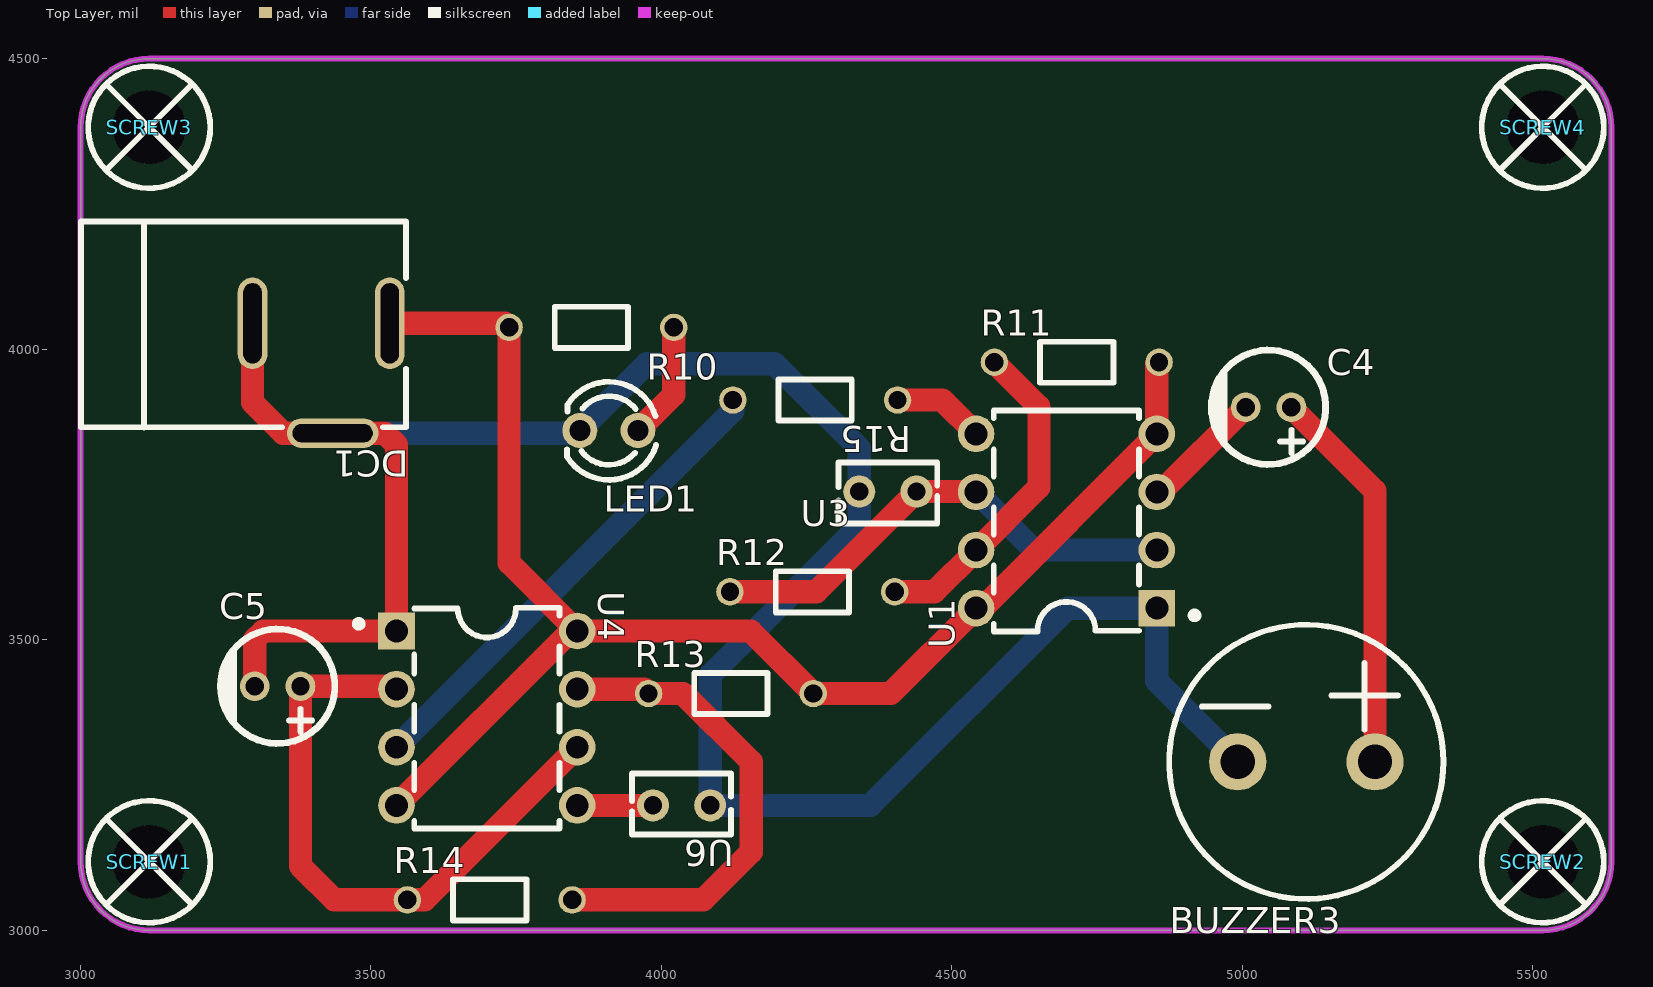
[diagram p0: Top Layer view]
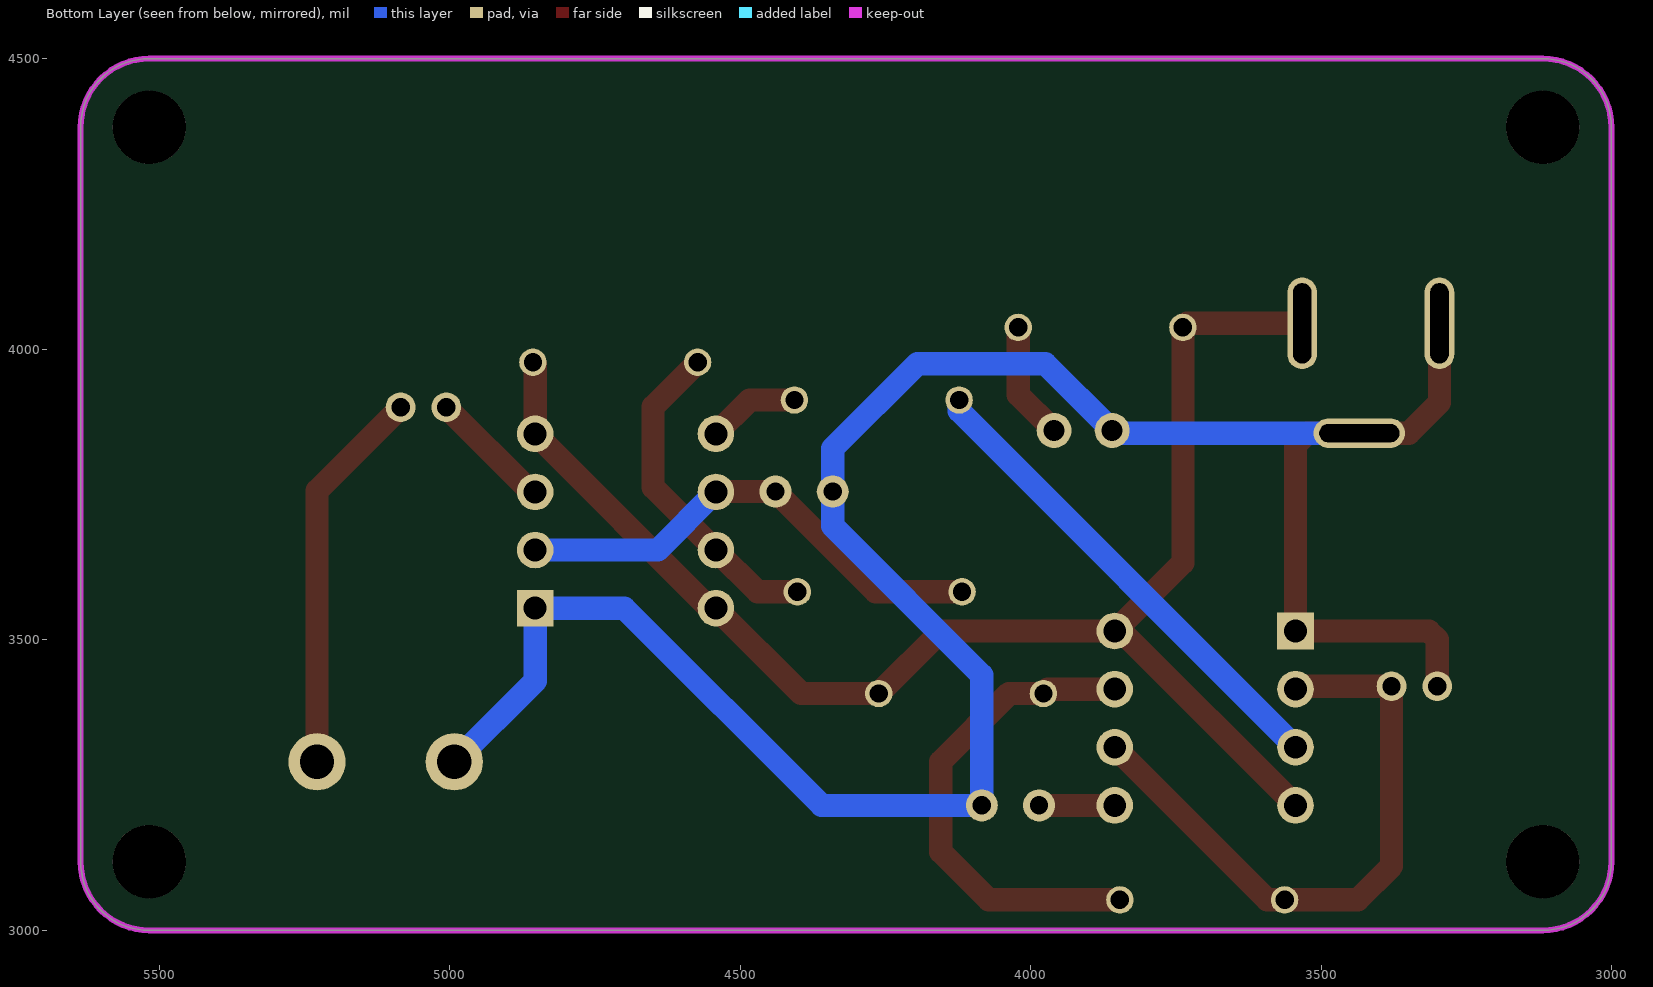
[diagram p1: Bottom Layer view, seen from below]
# Altium PCB MISC51829.pcbdoc
Units mil, origin at the board's own origin, x right, y up, seen from the top; angles counter-clockwise.
Board outline 2634.02 x 1500 mil, 2 copper layers (Top Layer, Bottom Layer), stack 62.206 mil thick; 19 components, 12 nets, 47 pads, 0 vias.

## Layer stack, top to bottom
Top Solder Mask Layer: solder mask 0.394, Dk 3.3
Top Layer: signal copper 1.379
Dielectric1: surface 59.449, FR4, Dk 4.5
Bottom Layer: signal copper 1.378
Bottom Solder Mask Layer: solder mask 0.394, Dk 3.3

## Board outline
3119.09,4500 ccw(c3119.09,4381.89) 3000.98,4381.89 3000.98,3118.11 ccw(c3119.09,3118.11) 3119.09,3000 5516.89,3000 ccw(c5516.89,3118.11) 5635,3118.11 5635,4381.89 ccw(c5516.89,4381.89) 5516.89,4500

## Design rules (kind name [scope] priority, off if disabled: settings)
BoardOutlineClearance copperThickness2oz_1 [All] p2 off: genericclearance=7.99 ignorepadtopadclearanceinfootprint=FALSE except(0: Arc-SplitContinuation Track-SplitContinuation SMDPad-SplitContinuation THPad-SplitContinuation Via-SplitContinuation Fill-SplitContinuation Region-SplitContinuation Poly-SplitContinuation Text-SplitContinuation Hole-SplitContinuation; 5.98: Arc-CutoutEdge Track-CutoutEdge SMDPad-CutoutEdge THPad-CutoutEdge Via-CutoutEdge Text-CutoutEdge; 6.9: Hole-OutlineEdge Hole-CutoutEdge; 10: Poly-OutlineEdge Poly-CutoutEdge; 11.81: Arc-OutlineEdge Track-OutlineEdge SMDPad-OutlineEdge THPad-OutlineEdge Via-OutlineEdge Fill-OutlineEdge Region-OutlineEdge Text-OutlineEdge Fill-CutoutEdge Region-CutoutEdge)
BoardOutlineClearance Plane_innerPlane_1 [All] p4 off: genericclearance=4.02 ignorepadtopadclearanceinfootprint=FALSE except(0: Arc-SplitContinuation Track-SplitContinuation SMDPad-SplitContinuation THPad-SplitContinuation Via-SplitContinuation Fill-SplitContinuation Region-SplitContinuation Poly-SplitContinuation Text-SplitContinuation Hole-SplitContinuation; 5.98: Arc-CutoutEdge Track-CutoutEdge SMDPad-CutoutEdge THPad-CutoutEdge Via-CutoutEdge Text-CutoutEdge; 6.9: Hole-OutlineEdge Hole-CutoutEdge; 10: Poly-OutlineEdge Poly-CutoutEdge; 11.81: Arc-OutlineEdge Track-OutlineEdge SMDPad-OutlineEdge THPad-OutlineEdge Via-OutlineEdge Fill-OutlineEdge Region-OutlineEdge Text-OutlineEdge Fill-CutoutEdge Region-CutoutEdge)
BoardOutlineClearance Copper_copperRegion_1 [All] p6 off: genericclearance=4.02 ignorepadtopadclearanceinfootprint=FALSE except(0: Arc-SplitContinuation Track-SplitContinuation SMDPad-SplitContinuation THPad-SplitContinuation Via-SplitContinuation Fill-SplitContinuation Region-SplitContinuation Poly-SplitContinuation Text-SplitContinuation Hole-SplitContinuation; 5.98: Arc-CutoutEdge Track-CutoutEdge SMDPad-CutoutEdge THPad-CutoutEdge Via-CutoutEdge Text-CutoutEdge; 6.9: Hole-OutlineEdge Hole-CutoutEdge; 10: Poly-OutlineEdge Poly-CutoutEdge; 11.81: Arc-OutlineEdge Track-OutlineEdge SMDPad-OutlineEdge THPad-OutlineEdge Via-OutlineEdge Fill-OutlineEdge Region-OutlineEdge Text-OutlineEdge Fill-CutoutEdge Region-CutoutEdge)
BoardOutlineClearance copperThickness1oz_1 [All] p8: genericclearance=4.02 ignorepadtopadclearanceinfootprint=FALSE except(0: Arc-SplitContinuation Track-SplitContinuation SMDPad-SplitContinuation THPad-SplitContinuation Via-SplitContinuation Fill-SplitContinuation Region-SplitContinuation Poly-SplitContinuation Text-SplitContinuation Hole-SplitContinuation; 5.98: Arc-CutoutEdge Track-CutoutEdge SMDPad-CutoutEdge THPad-CutoutEdge Via-CutoutEdge Text-CutoutEdge; 6.9: Hole-OutlineEdge Hole-CutoutEdge; 10: Poly-OutlineEdge Poly-CutoutEdge; 11.81: Arc-OutlineEdge Track-OutlineEdge SMDPad-OutlineEdge THPad-OutlineEdge Via-OutlineEdge Fill-OutlineEdge Region-OutlineEdge Text-OutlineEdge Fill-CutoutEdge Region-CutoutEdge)
Clearance copperThickness2oz [All] p1 off: gap=7.99 ignorepadtopadclearanceinfootprint=FALSE except(5.98: SMDPad-Track SMDPad-SMDPad THPad-Track SMDPad-THPad THPad-THPad Track-Via SMDPad-Via THPad-Via Via-Via Fill-SMDPad Region-SMDPad Fill-THPad Region-THPad Fill-Via Region-Via Fill-Fill Fill-Region Region-Region Arc-Track Arc-SMDPad Arc-THPad Arc-Via Fill-Arc Region-Arc Arc-Arc Text-Track SMDPad-Text Text-THPad Text-Via Fill-Text Region-Text Arc-Text Text-Text; 6.9: Hole-Track Hole-SMDPad Hole-THPad Hole-Via Fill-Hole Region-Hole Hole-Arc Hole-Text; 10: Poly-Track Poly-SMDPad Poly-THPad Poly-Via Poly-Fill Poly-Region Poly-Poly Poly-Arc Poly-Text Poly-Hole; 11.81: Fill-Track Region-Track)
Clearance Plane_innerPlane [All] p3 off: gap=4.02 ignorepadtopadclearanceinfootprint=FALSE except(5.98: SMDPad-Track SMDPad-SMDPad THPad-Track SMDPad-THPad THPad-THPad Track-Via SMDPad-Via THPad-Via Via-Via Fill-SMDPad Region-SMDPad Fill-THPad Region-THPad Fill-Via Region-Via Fill-Fill Fill-Region Region-Region Arc-Track Arc-SMDPad Arc-THPad Arc-Via Fill-Arc Region-Arc Arc-Arc Text-Track SMDPad-Text Text-THPad Text-Via Fill-Text Region-Text Arc-Text Text-Text; 6.9: Hole-Track Hole-SMDPad Hole-THPad Hole-Via Fill-Hole Region-Hole Hole-Arc Hole-Text; 10: Poly-Track Poly-SMDPad Poly-THPad Poly-Via Poly-Fill Poly-Region Poly-Poly Poly-Arc Poly-Text Poly-Hole; 11.81: Fill-Track Region-Track)
Clearance Copper_copperRegion [All] p5 off: gap=4.02 ignorepadtopadclearanceinfootprint=FALSE except(5.98: SMDPad-Track SMDPad-SMDPad THPad-Track SMDPad-THPad THPad-THPad Track-Via SMDPad-Via THPad-Via Via-Via Fill-SMDPad Region-SMDPad Fill-THPad Region-THPad Fill-Via Region-Via Fill-Fill Fill-Region Region-Region Arc-Track Arc-SMDPad Arc-THPad Arc-Via Fill-Arc Region-Arc Arc-Arc Text-Track SMDPad-Text Text-THPad Text-Via Fill-Text Region-Text Arc-Text Text-Text; 6.9: Hole-Track Hole-SMDPad Hole-THPad Hole-Via Fill-Hole Region-Hole Hole-Arc Hole-Text; 10: Poly-Track Poly-SMDPad Poly-THPad Poly-Via Poly-Fill Poly-Region Poly-Poly Poly-Arc Poly-Text Poly-Hole; 11.81: Fill-Track Region-Track)
Clearance copperThickness1oz [All] p7: gap=4.02 ignorepadtopadclearanceinfootprint=FALSE except(5.98: SMDPad-Track SMDPad-SMDPad THPad-Track SMDPad-THPad THPad-THPad Track-Via SMDPad-Via THPad-Via Via-Via Fill-SMDPad Region-SMDPad Fill-THPad Region-THPad Fill-Via Region-Via Fill-Fill Fill-Region Region-Region Arc-Track Arc-SMDPad Arc-THPad Arc-Via Fill-Arc Region-Arc Arc-Arc Text-Track SMDPad-Text Text-THPad Text-Via Fill-Text Region-Text Arc-Text Text-Text; 6.9: Hole-Track Hole-SMDPad Hole-THPad Hole-Via Fill-Hole Region-Hole Hole-Arc Hole-Text; 10: Poly-Track Poly-SMDPad Poly-THPad Poly-Via Poly-Fill Poly-Region Poly-Poly Poly-Arc Poly-Text Poly-Hole; 11.81: Fill-Track Region-Track)
DiffPairsRouting differentialPair [All] p1: maxlimit=6 minlimit=6 mostfreqgap=6 toplayer_minwidth=5 toplayer_prefwidth=10 toplayer_maxwidth=100 toplayer_mingap=6 toplayer_prefgap=6 toplayer_maxgap=6 bottomlayer_minwidth=5 bottomlayer_prefwidth=10 bottomlayer_maxwidth=100 bottomlayer_mingap=6 bottomlayer_prefgap=6 bottomlayer_maxgap=6 maxuncoupledlength=10
HoleToHoleClearance otherClearance [All] p1: gap=11.81 allowstackedmicrovias=TRUE
Length netLength [All] p1: minlimit=0 maxlimit=0
PasteMaskExpansion pasteMaskExpansion [All] p1: expansion=0
PlaneConnect innerPlane [All] p1: planeconnectstyle=Relief reliefexpansion=20 reliefentries=4 reliefconductorwidth=10 reliefairgap=10
PolygonConnect copperRegion [All] p1: connectstyle=Relief reliefconductorwidth=10 reliefentries=4 polygonreliefangle="90 Angle" airgapwidth=10 via.connectstyle=Relief via.reliefconductorwidth=10 via.reliefentries=4 via.polygonreliefangle="90 Angle" via.airgapwidth=10
RoutingVias viaSize [All] p1: holewidth=12.01 width=24.02 viastyle="Through Hole" minholewidth=11.81 minwidth=19.68 maxholewidth=248.03 maxwidth=393.7
SolderMaskExpansion solderMaskExpansion [IsVia] p1: expansion=-1000 istentingtop=TRUE
SolderMaskExpansion solderMaskExpansion [All] p2: expansion=2 istentingtop=FALSE
Width copperThickness2oz_2 [All] p1 off: maxlimit=100 minlimit=8 preferedwidth=10
Width copperThickness1oz_2 [All] p2: maxlimit=100 minlimit=5 preferedwidth=10

## Components (designator, comment, footprint, x,y, rotation, side; value= is the part's Value field where it differs from the comment)
BUZZER3 "buzzer" BUZ-TH_BD12.0-P6.00-D0.9-RD 5110,3290 r0 top
C4 "10uF" CAP-TH_BD5.0-P2.00-D0.8-FD 5045,3900 r180 top
C5 "47uF" CAP-TH_BD5.0-P2.00-D0.8-FD 3340,3420 r180 top
DC1 "" DC-2.0 3410,4055 r180 top
LED1 "" LED_TH-3mm 3910,3860 r180 top
R10 "1kΩ" Res_1/8W 3880,4040 r180 top
R11 "4.7kΩ" Res_1/8W 4715,3975 r0 top
R12 "6.8kΩ" Res_1/8W 4260,3580 r0 top
R13 "1kΩ" Res_1/8W 4120,3405 r0 top
R14 "15kΩ" Res_1/8W 3705,3050 r0 top
R15 "5.1kΩ" Res_1/8W 4265,3915 r180 top
SCREW1 "" M3螺丝 3119.09,3118.11 r0 top
SCREW2 "" M3螺丝 5516.89,3118.11 r0 top
SCREW3 "" M3螺丝 3119.09,4381.89 r0 top
SCREW4 "" M3螺丝 5516.89,4381.89 r0 top
U1 "NE555" PDIP-8_L9.6-W6.4-P2.54-LS7.9-BL-1 4697.34,3704.34 r90 top
U3 "100nF" CAP-TH_L4.0-W2.5-P2.50-D0.5 4390,3755 r0 top
U4 "NE555" PDIP-8_L9.6-W6.4-P2.54-LS7.9-BL-1 3700,3365 r270 top
U6 "10nF" CAP-TH_L4.0-W2.5-P2.50-D0.5 4035,3215 r180 top

## Footprints (in the part's own frame and the unit in brackets; to place one, negate y for a bottom-side part, rotate by r counter-clockwise, add the part's x,y. Pads: shape width x height; smd on the part's side, far side on the other; paste and mask are expansions set on the pad)
BUZ-TH_BD12.0-P6.00-D0.9-RD [mm]
  round 2.5 hole 1.5 paste+0 mask+0.05: 1(-3,0) 2(3,0)
  silkscreen extent -5.99,-5.99 5.99,5.99
CAP-TH_BD5.0-P2.00-D0.8-FD [mm]
  round 1.3 hole 0.8: 1(-1,0) 2(1,0)
  silkscreen extent -2.5,-2.5 2.5,2.5
CAP-TH_L4.0-W2.5-P2.50-D0.5 [mm]
  round 1.4 hole 0.8 paste+0 mask+0.05: 1(-1.25,0) 2(1.25,0)
  silkscreen extent -2.16,-1.4 2.16,1.27
DC-2.0 [mil]
  oval 157.5x51.2 hole 31.5 slot 137.8 at 0 deg paste+0 mask+2: 2(-24.7,199.5)
  oval 51.2x157.5 hole 31.5 slot 137.8 at 90 deg paste+0 mask+2: 3(113.1,10.5) 4(-123.1,10.5)
  silkscreen extent -151,-165 408,190
LED_TH-3mm [mil]
  round 60 hole 36 paste+0 mask+2: 1(-50,0) 2(50,0)
  silkscreen extent -81,-84 72,85
M3螺丝 [mil]
  round 126 hole 126 paste+0 mask+4: 1(0,0)
  silkscreen extent -105,-105 105,105
PDIP-8_L9.6-W6.4-P2.54-LS7.9-BL-1 [mil]
  rect 63x63 hole 39.37: 1(-150,-155.51)
  round 63 hole 39.37: 2(-50,-155.51) 3(50,-155.51) 4(150,-155.51) 5(150,155.52) 6(50,155.52) 7(-50,155.52) 8(-150,155.52)
  silkscreen extent -190,-226 190,125
Res_1/8W [mil]
  round 47.2 hole 31.5 paste+0 mask+2: 1(-141.7,2.48) 2(141.7,2.48)
  silkscreen extent -63,-33 63,38

## Nets (pads, with @x,y where several pads share a name; then routed paths per layer and width w, separated by ;. In a path a pad name is that pad's centre, name@x,y a point inside that pad or via, vN(x,y) a via of type N, cw(c..) or ccw(c..) an arc to the next point about the centre after c; other vN are vias at no path point)
$1N4636: LED1.1 R10.1 | length 203.1
  Top Layer w40: LED1.1 4021.7,3921.7 R10.1
$1N5933: C4.2 U1.3 | length 213.1
  Top Layer w40: U1.3 4859.97,3754.34 C4.2
$1N5936: R11.1 R12.2 U1.7 | length 569.6
  Top Layer w40: R12.2 4469.96,3582.48 U1.7 4650,3762.52 4650,3900.78 R11.1
$1N5938: R12.1 U1.2 U1.6 U3.2 | length 847.7
  Top Layer w40: R12.1 4266.69,3582.48 U3.2 4541.17,3755 U1.6
  Bottom Layer w40: U1.6 4641.83,3654.34 U1.2
$1N5940: BUZZER3.2 C4.1 | length 669.5
  Top Layer w40: C4.1 5228.11,3756.26 BUZZER3.2
$1N5995: R15.1 U1.5 | length 159.2
  Top Layer w40: R15.1 4483.65,3912.52 U1.5
$1N6290: C5.1 R14.1 U4.2 U4.6 | length 1085.5
  Top Layer w40: U4.2 3539.49,3420 C5.1 3379.37,3110.63 3437.52,3052.48 R14.1 3592.99,3052.48 U4.6
$1N6296: R13.1 R14.2 U4.7 | length 848.7
  Top Layer w40: R14.2 4072.48,3052.48 4155,3135 4155,3290 4037.52,3407.48 R13.1 3970.78,3415 U4.7
$1N6341: R15.2 U4.3 | length 837.3
  Bottom Layer w40: U4.3 4123.3,3893.81 R15.2
$1N6358: U4.5 U6.2 | length 130.3
  Top Layer w40: U4.5 U6.2
+5V: DC1.4 R10.2 R11.2 R13.2 U1.4 U1.8 U4.4 U4.8 | length 2566.1
  Top Layer w40: DC1.4 3731.32,4044.5 R10.2 3738.3,3632.21 U4.8 ; U4.4 3844.49,3515 U4.8 ; R11.2 4852.85,3973.62 U1.4 4552.85,3554.34 U1.8 4394.96,3407.48 R13.2 4154.18,3515 U4.8
GND: BUZZER3.1 C5.2 DC1.2 DC1.3 LED1.2 U1.1 U3.1 U4.1 U6.1 | length 4032.6
  Top Layer w40: DC1.3 3296.9,3908.1 3349.5,3855.5 DC1.2 3524.5,3855.5 3544.49,3835.51 U4.1 3315,3515 3300.63,3500.63 C5.2
  Bottom Layer w40: DC1.2 3855.5,3855.5 LED1.2 3975,3975 4195,3975 4340.79,3829.21 U3.1 4340.79,3695.79 4084.21,3439.21 U6.1 4360,3215 4699.34,3554.34 U1.1 4852.85,3429.04 BUZZER3.1
pads on no net: SCREW1.1 SCREW2.1 SCREW3.1 SCREW4.1

## Keep-outs
Board Outline Layer:
  the board outline again, w10